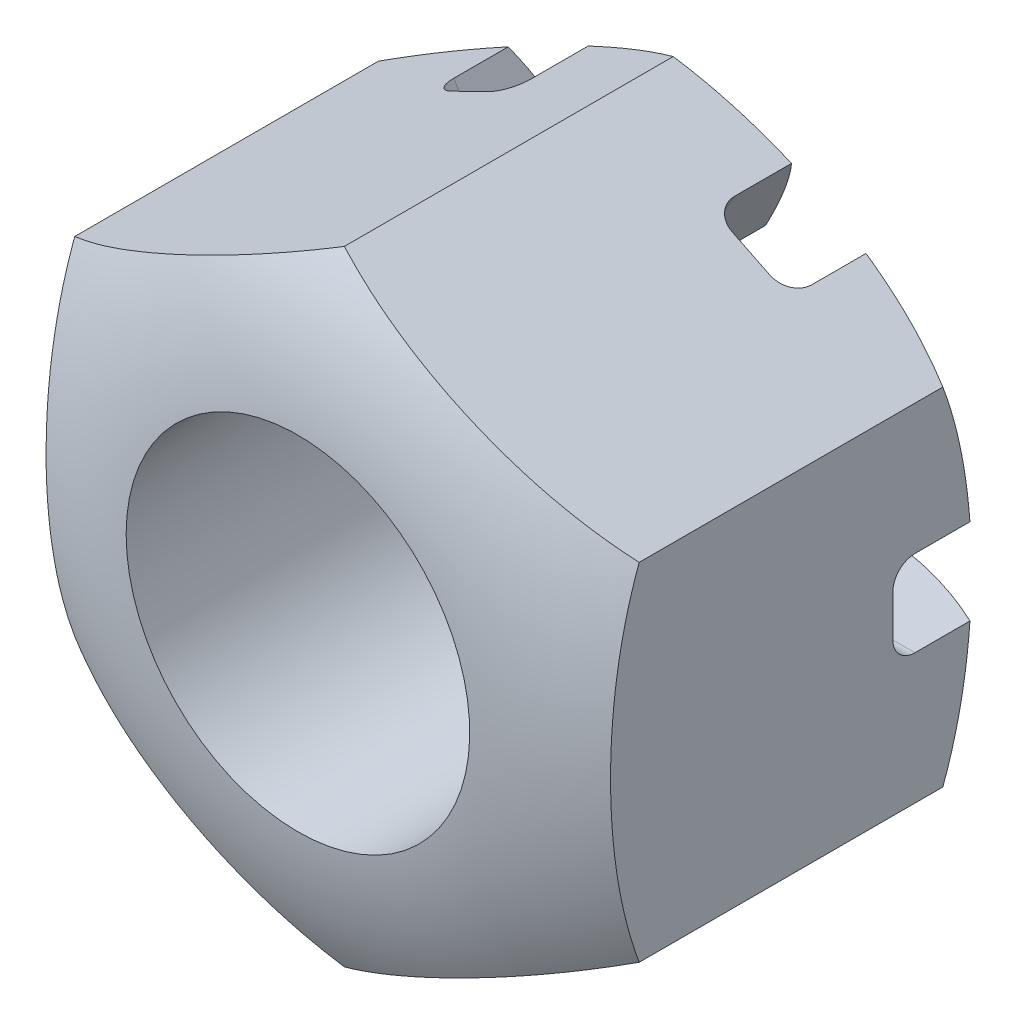
from build123d import *

# Parameters (mm, degrees)
EXTRUDE_1_DEPTH          = 34.6
SKETCH_3_W               = 65
SKETCH_3_H               = 7
CUT_EXTRUDE_1_DEPTH      = 9
PATTERN_CIRCULAR_1_COUNT = 3
PATTERN_CIRCULAR_1_ANGLE = 120
M30X2_0_1_D              = 28
FILLET_2_R               = 1.8


with BuildPart() as part:
    # 草图1 → 凸台-拉伸1 (new body)
    with BuildSketch(Plane.XY):
        Polygon((0, 25.425), (-23.00014754, 14.1137269), (-23.00014754, -14.1137269), (0, -25.425), (23.00014754, -14.1137269), (23.00014754, 14.1137269), align=None)
    extrude(amount=EXTRUDE_1_DEPTH)

    # 草图3 → 切除-拉伸1 (cut)
    with BuildSketch(Plane(origin=(0, 0, 0), x_dir=(-1, 0, 0), z_dir=(0, 0, -1))):
        Rectangle(SKETCH_3_W, SKETCH_3_H)
    cut_extrude_1 = extrude(amount=-CUT_EXTRUDE_1_DEPTH, mode=Mode.SUBTRACT)

    # 阵列(圆周)1: 切除-拉伸1 ×3 about axis
    pattern_circular_1_axis = Axis((0, 0, 0), (0, 0, 1))
    for i in range(1, PATTERN_CIRCULAR_1_COUNT):
        add(cut_extrude_1.rotate(pattern_circular_1_axis, i * PATTERN_CIRCULAR_1_ANGLE / (PATTERN_CIRCULAR_1_COUNT - 1)), mode=Mode.SUBTRACT)

    # M30x2.0 螺纹孔1 (through all)
    with Locations(Plane.XY.offset(34.6)):
        with Locations((0, 0)):
            Hole(M30X2_0_1_D / 2)

    # 圆角2
    fillet_2_edges = [part.edges().sort_by_distance(p)[0] for p in [
        (-12.194715533, 14.121866887, 9),
        (6.015921174, 17.419881127, 9),
        (-6.015921174, -17.419881127, 9),
        (12.194715533, -14.121866887, 9),
        (-18.277794626, -3.5, 9),
        (18.277794626, 3.5, 9),
        (-18.277794626, 3.5, 9),
        (18.277794626, -3.5, 9),
        (-6.015921174, 17.419881127, 9),
        (6.015921174, -17.419881127, 9),
        (12.194715533, 14.121866887, 9),
        (-12.194715533, -14.121866887, 9),
    ]]
    fillet(fillet_2_edges, radius=FILLET_2_R)

    # 草图8 → 切除-旋转1 (revolve, cut)
    with BuildSketch(Plane(origin=(0, 0, 0), x_dir=(1, 0, 0), z_dir=(0, 1, 0)), mode=Mode.PRIVATE) as cut_revolve_1_sk:
        with BuildLine():
            Line((11.5, 0), (33.520524336, 0))
            Line((33.520524336, 0), (33.520524336, -11.524643769))
            ThreePointArc((33.520524336, -11.524643769), (23.926995876, -3.055321154), (11.5, 0))
        make_face()
        with BuildLine():
            Line((11.5, -34.6), (33.520524336, -34.6))
            Line((33.520524336, -34.6), (33.520524336, -23.075356231))
            ThreePointArc((33.520524336, -23.075356231), (23.926995876, -31.544678846), (11.5, -34.6))
        make_face()
    revolve(cut_revolve_1_sk.sketch.rotate(Axis((0, 0, -1.73), (0, 0, 1)), 353.025443337), axis=Axis((0, 0, -1.73), (0, 0, 1)), mode=Mode.SUBTRACT)


solid = part.part
